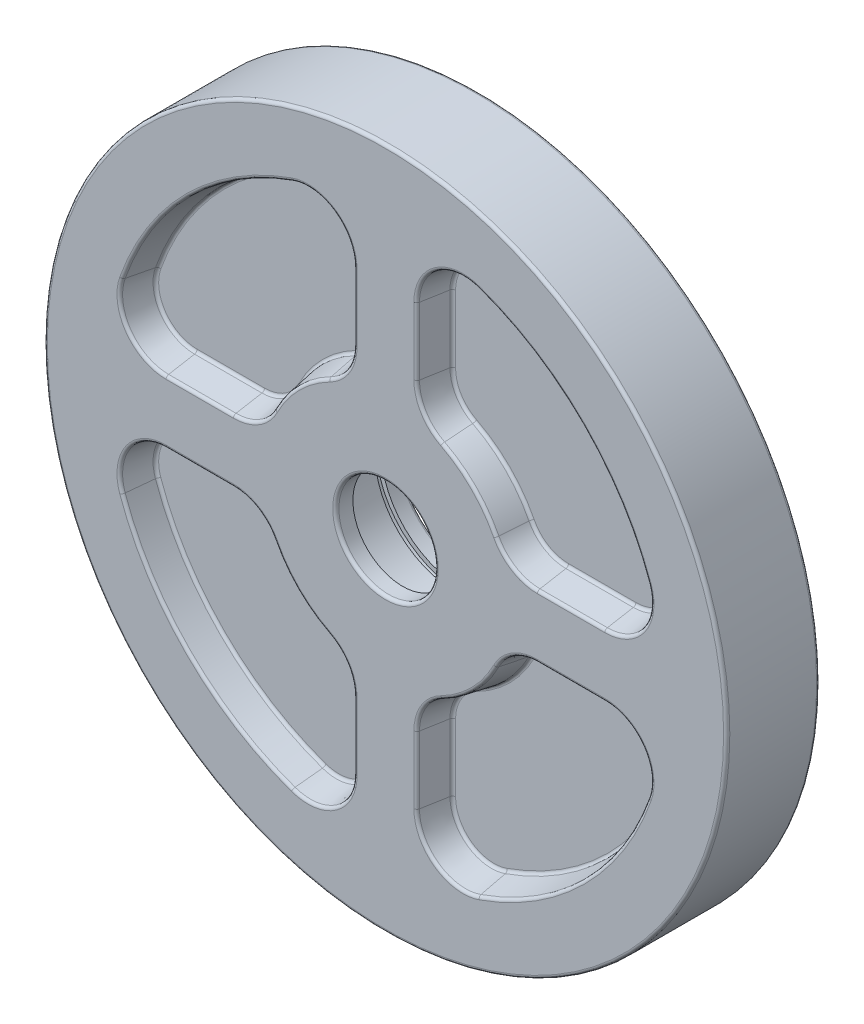
SolidWorks part; units mm, degrees
ref_plane "Front Plane" through (0, 0, 0) normal (0, 0, 1) x (1, 0, 0)
ref_plane "Top Plane" through (0, 0, 0) normal (0, 1, 0) x (1, 0, 0)
ref_plane "Right Plane" through (0, 0, 0) normal (1, 0, 0) x (0, 0, -1)
sketch "Sketch1" plane through (0, 0, 0) normal (0, 0, 1) x (1, 0, 0)
  circle A0 centre (0, 0) radius 110
  dimension "D1" = 220
extrude "Boss-Extrude1" add sketch "Sketch1" along normal mid plane 30
sketch "Sketch2" plane through (0, 0, 15) normal (0, 0, 1) x (1, 0, 0)
  circle A0 centre (0, 0) radius 16
  dimension "D1" = 32
extrude "Cut-Extrude1" cut sketch "Sketch2" against normal blind 5.5
sketch "Sketch3" plane through (0, 0, 9.5) normal (0, 0, 1) x (1, 0, 0)
  circle A0 centre (0, 0) radius 22.5
  dimension "D1" = 45
extrude "Cut-Extrude2" cut sketch "Sketch3" against normal blind 2
sketch "Sketch4" plane through (0, 0, 7.5) normal (0, 0, 1) x (1, 0, 0)
  circle A0 centre (0, 0) radius 26
  dimension "D1" = 52
extrude "Cut-Extrude3" cut sketch "Sketch4" against normal blind 15
sketch "Sketch5" plane through (0, 0, -7.5) normal (0, 0, 1) x (1, 0, 0)
  circle A0 centre (0, 0) radius 27.5
  dimension "D1" = 55
extrude "Cut-Extrude4" cut sketch "Sketch5" against normal blind 2
sketch "Sketch6" plane through (0, 0, -9.5) normal (0, 0, 1) x (1, 0, 0)
  circle A0 centre (0, 0) radius 26
  dimension "D1" = 52
extrude "Cut-Extrude5" cut sketch "Sketch6" against normal through all
sketch "Sketch7" plane through (0, 0, -15) normal (0, 0, -1) x (-1, 0, 0)
  line L1 (-10, 70.7107) -> (-10, 48.9898)
  line L7 (-70.7107, 10) -> (-48.9898, 10)
  arc A0 (-18.1818, 35.6289) -> (-35.6289, 18.1818) centre (0, 0) ccw
  arc A1 (-30, 84.8528) -> (-84.8528, 30) centre (0, 0) ccw
  arc A2 (-35.6289, 18.1818) -> (-48.9898, 10) centre (-48.9898, 25) cw
  arc A3 (-84.8528, 30) -> (-70.7107, 10) centre (-70.7107, 25) ccw
  arc A4 (-18.1818, 35.6289) -> (-10, 48.9898) centre (-25, 48.9898) ccw
  arc A5 (-10, 70.7107) -> (-30, 84.8528) centre (-25, 70.7107) ccw
  point P4 (0, 101.8147)
  point P5 (0, 31.4133)
  point P6 (-10, 101.8147)
  point P7 (-10, 31.4133)
  point P8 (10, 101.8147)
  point P9 (10, 31.4133)
  point P28 (0, 0)
  dimension "D1" = 80
  dimension "D2" = 180
  dimension "D3" = 15
extrude "Cut-Extrude6" cut sketch "Sketch7" against normal blind 10 draft 10
pattern_circular "CirPattern1" count 4 over 360 about axis through (0, 0, 0) along (0, 0, 1) of "Cut-Extrude6"
mirror "Mirror1" about plane through (0, 0, 0) normal (0, 0, 1) of "CirPattern1", "Cut-Extrude6"
fillet "Fillet1" radius 1 66 edges at (59.8502, 11.7633, -5) (81.5184, 17.3578, -5) (62.3928, 62.3928, -5) (17.3578, 81.5184, -5) (11.7633, 59.8502, -5) (13.7117, 42.0771, -5) (29.5311, 29.5311, -5) (42.0771, 13.7117, -5) (11.7633, -59.8502, -5) (17.3578, -81.5184, -5) (62.3928, -62.3928, -5) (81.5184, -17.3578, -5) (59.8502, -11.7633, -5) (42.0771, -13.7117, -5) (29.5311, -29.5311, -5) (13.7117, -42.0771, -5) (-59.8502, -11.7633, -5) (-81.5184, -17.3578, -5) (-62.3928, -62.3928, -5) (-17.3578, -81.5184, -5) (-11.7633, -59.8502, -5) (-13.7117, -42.0771, -5) (-29.5311, -29.5311, -5) (-42.0771, -13.7117, -5) (-11.7633, 59.8502, -5) (-17.3578, 81.5184, -5) (-62.3928, 62.3928, -5) (-81.5184, 17.3578, -5) (-59.8502, 11.7633, -5) (-42.0771, 13.7117, -5) (-29.5311, 29.5311, -5) (-13.7117, 42.0771, -5) (110, 0, -15) (26, 0, -15) (12.208, 41.1563, -15) (10, 59.8502, -15) (16.3397, 82.9581, -15) (63.6396, 63.6396, -15) (82.9581, 16.3397, -15) (59.8502, 10, -15) (41.1563, 12.208, -15) (28.2843, 28.2843, -15) (41.1563, -12.208, -15) (59.8502, -10, -15) (82.9581, -16.3397, -15) (63.6396, -63.6396, -15) (16.3397, -82.9581, -15) (10, -59.8502, -15) (12.208, -41.1563, -15) (28.2843, -28.2843, -15) (-12.208, -41.1563, -15) (-10, -59.8502, -15) (-16.3397, -82.9581, -15) (-63.6396, -63.6396, -15) (-82.9581, -16.3397, -15) (-59.8502, -10, -15) (-41.1563, -12.208, -15) (-28.2843, -28.2843, -15) (-41.1563, 12.208, -15) (-59.8502, 10, -15) (-82.9581, 16.3397, -15) (-63.6396, 63.6396, -15) (-16.3397, 82.9581, -15) (-10, 59.8502, -15) (-12.208, 41.1563, -15) (-28.2843, 28.2843, -15)
fillet "Fillet2" radius 1 66 edges at (-29.5311, -29.5311, 5) (-13.7117, -42.0771, 5) (-11.7633, -59.8502, 5) (-17.3578, -81.5184, 5) (-62.3928, -62.3928, 5) (-81.5184, -17.3578, 5) (-59.8502, -11.7633, 5) (-42.0771, -13.7117, 5) (29.5311, -29.5311, 5) (42.0771, -13.7117, 5) (59.8502, -11.7633, 5) (81.5184, -17.3578, 5) (62.3928, -62.3928, 5) (17.3578, -81.5184, 5) (11.7633, -59.8502, 5) (13.7117, -42.0771, 5) (29.5311, 29.5311, 5) (13.7117, 42.0771, 5) (11.7633, 59.8502, 5) (17.3578, 81.5184, 5) (62.3928, 62.3928, 5) (81.5184, 17.3578, 5) (59.8502, 11.7633, 5) (42.0771, 13.7117, 5) (-29.5311, 29.5311, 5) (-42.0771, 13.7117, 5) (-59.8502, 11.7633, 5) (-81.5184, 17.3578, 5) (-62.3928, 62.3928, 5) (-17.3578, 81.5184, 5) (-11.7633, 59.8502, 5) (-13.7117, 42.0771, 5) (-16.3397, 82.9581, 15) (-63.6396, 63.6396, 15) (-82.9581, 16.3397, 15) (-59.8502, 10, 15) (-41.1563, 12.208, 15) (-28.2843, 28.2843, 15) (-12.208, 41.1563, 15) (-10, 59.8502, 15) (16.3397, -82.9581, 15) (63.6396, -63.6396, 15) (82.9581, -16.3397, 15) (59.8502, -10, 15) (41.1563, -12.208, 15) (28.2843, -28.2843, 15) (12.208, -41.1563, 15) (10, -59.8502, 15) (110, 0, 15) (16, 0, 15) (82.9581, 16.3397, 15) (63.6396, 63.6396, 15) (16.3397, 82.9581, 15) (10, 59.8502, 15) (12.208, 41.1563, 15) (28.2843, 28.2843, 15) (41.1563, 12.208, 15) (59.8502, 10, 15) (-82.9581, -16.3397, 15) (-63.6396, -63.6396, 15) (-16.3397, -82.9581, 15) (-10, -59.8502, 15) (-12.208, -41.1563, 15) (-28.2843, -28.2843, 15) (-41.1563, -12.208, 15) (-59.8502, -10, 15)
sketch "Sketch8" plane through (0, 0, -15) normal (0, 0, -1) x (-1, 0, 0)
  circle A1 centre (0, 32.5) radius 1.5
  circle A2 centre (28.1458, -16.25) radius 1.5
  circle A3 centre (-28.1458, -16.25) radius 1.5
  point P11 (0, 0)
  dimension "D2" = 3
  dimension "D3" = 3
extrude "Cut-Extrude7" cut sketch "Sketch8" against normal blind 10
